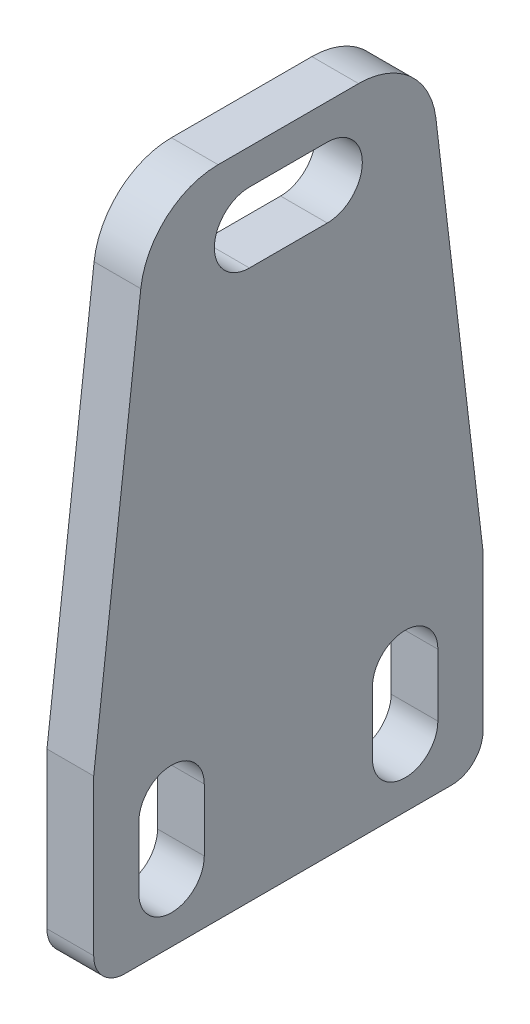
SolidWorks part; units mm, degrees
material "不锈钢201"
ref_plane "前视基准面" through (0, 0, 0) normal (0, 0, 1) x (1, 0, 0)
ref_plane "上视基准面" through (0, 0, 0) normal (0, 1, 0) x (1, 0, 0)
ref_plane "右视基准面" through (0, 0, 0) normal (1, 0, 0) x (0, 0, -1)
sketch "草图1" plane through (0, 0, 0) normal (1, 0, 0) x (0, 0, -1)
  line L0 (0, 33.5) -> (0, -7.9603) construction
  line L1 (-12.5, 6) -> (-6, 6)
  line L2 (-12.5, 6) -> (-12.5, -6)
  line L3 (-12.5, -6) -> (12.5, -6)
  line L4 (12.5, 6) -> (12.5, -6)
  line L5 (-12.5, 6) -> (12.5, -6) construction
  line L6 (-12.5, -6) -> (12.5, 6) construction
  line L7 (-6, 61) -> (6, 61)
  line L8 (-6, 61) -> (-6, 6)
  line L10 (6, 61) -> (6, 6)
  line L11 (-6, 61) -> (6, 6) construction
  line L12 (-6, 6) -> (6, 61) construction
  line L14 (6, 6) -> (12.5, 6)
  point P0 (0, 0)
  point P6 (0, 33.5)
  dimension "D1" = 12
  dimension "D2" = 25
  dimension "D3" = 12
  dimension "D4" = 55
extrude "凸台-拉伸1" add sketch "草图1" along normal blind 3
sketch "草图2" plane through (0, 0, 0) normal (-1, 0, 0) x (0, 0, 1)
  line L0 (-6, 61) -> (-12.5, 6)
  line L1 (6, 61) -> (12.5, 6)
  line L2 (-6, 61) -> (6, 61)
  line L3 (-12.5, 6) -> (12.5, 6)
extrude "凸台-拉伸2" add sketch "草图2" against normal up to surface (3 mm away) up to face at (3, 16.75, 0)
fillet "圆角1" radius 2 2 edges at (1.5, 61, 6) (1.5, 61, -6)
sketch "草图3" plane through (0, 0, 0) normal (-1, 0, 0) x (0, 0, 1)
  line L0 (-9.6408, 0) -> (9.298, 0) construction
  line L1 (0, 0) -> (0, -6.9973) construction
  line L2 (-7.5, 2) -> (-7.5, -2) construction
  line L3 (-5.4, 2) -> (-5.4, -2)
  line L4 (-9.6, 2) -> (-9.6, -2)
  line L5 (7.5, 2) -> (7.5, -2) construction
  line L6 (5.4, 2) -> (5.4, -2)
  line L7 (9.6, 2) -> (9.6, -2)
  line L8 (12.5, -6) -> (-12.5, -6) construction
  arc A0 (-5.4, 2) -> (-9.6, 2) centre (-7.5, 2) ccw
  arc A1 (-9.6, -2) -> (-5.4, -2) centre (-7.5, -2) ccw
  arc A2 (5.4, 2) -> (9.6, 2) centre (7.5, 2) cw
  arc A3 (9.6, -2) -> (5.4, -2) centre (7.5, -2) cw
  point P7 (-7.5, 0)
  point P14 (7.5, 0)
  dimension "D4" = 2.1
  dimension "D1" = 15
  dimension "D2" = 4
  dimension "D3" = 6
extrude "切除-拉伸1" cut sketch "草图3" against normal blind 3
fillet "圆角2" radius 2 2 edges at (1.5, -6, -12.5) (1.5, -6, 12.5)
hole_wizard "Ø4.3 (4.3) 直径孔1" positions "草图4" profile "草图6" hole size "Ø4.3" standard "GB"
sketch "草图4" plane through (0, 0, 0) normal (-1, 0, 0) x (0, 0, 1)
  point P0 (0, 56)
  point P3 (0, 41)
sketch "草图6" plane through (0, 56, 0) normal (0, 1, 0) x (0, 0, 1)
  line L0 (0, 0) -> (0, 11.3919)
  line L1 (0, 11.3919) -> (2.15, 10.1)
  line L2 (2.15, 10.1) -> (2.15, 0)
  line L5 (2.15, 0) -> (0, 0)
  line L10 (0, 11.3919) -> (-2.15, 10.1) construction
  line L11 (0, -6.35) -> (0, 107.95) construction
  dimension "孔直径" = 4.3
  dimension "孔深度" = 10.1
  dimension "导头角度" = 118
sketch "草图7" plane through (3, 0, 0) normal (1, 0, 0) x (0, 0, -1)
  line L0 (4.2224, 61) -> (-4.2224, 61) construction
  line L1 (-13.476, 63.8853) -> (10.9733, 63.8853)
  line L2 (-13.476, 63.8853) -> (-13.476, 36)
  line L3 (-13.476, 36) -> (10.9733, 36)
  line L4 (10.9733, 63.8853) -> (10.9733, 36)
  dimension "D1" = 25
extrude "切除-拉伸2" cut sketch "草图7" against normal blind 10
sketch "草图8" plane through (0, 0, 0) normal (-1, 0, 0) x (0, 0, 1)
  line L0 (-2.5, 31.5) -> (2.5, 31.5) construction
  line L1 (-2.5, 33.75) -> (2.5, 33.75)
  line L2 (-2.5, 29.25) -> (2.5, 29.25)
  line L3 (8.9545, 36) -> (-8.9545, 36) construction
  line L4 (0, 0) -> (0, 48.2057) construction
  arc A0 (-2.5, 33.75) -> (-2.5, 29.25) centre (-2.5, 31.5) ccw
  arc A1 (2.5, 29.25) -> (2.5, 33.75) centre (2.5, 31.5) ccw
  point P2 (0, 31.5)
  point P12 (0, 0)
  dimension "D1" = 2.25
  dimension "D2" = 4.5
  dimension "D3" = 5
extrude "切除-拉伸3" cut sketch "草图8" against normal blind 10
fillet "圆角3" radius 5 2 edges at (1.5, 36, -8.9545) (1.5, 36, 8.9545)
